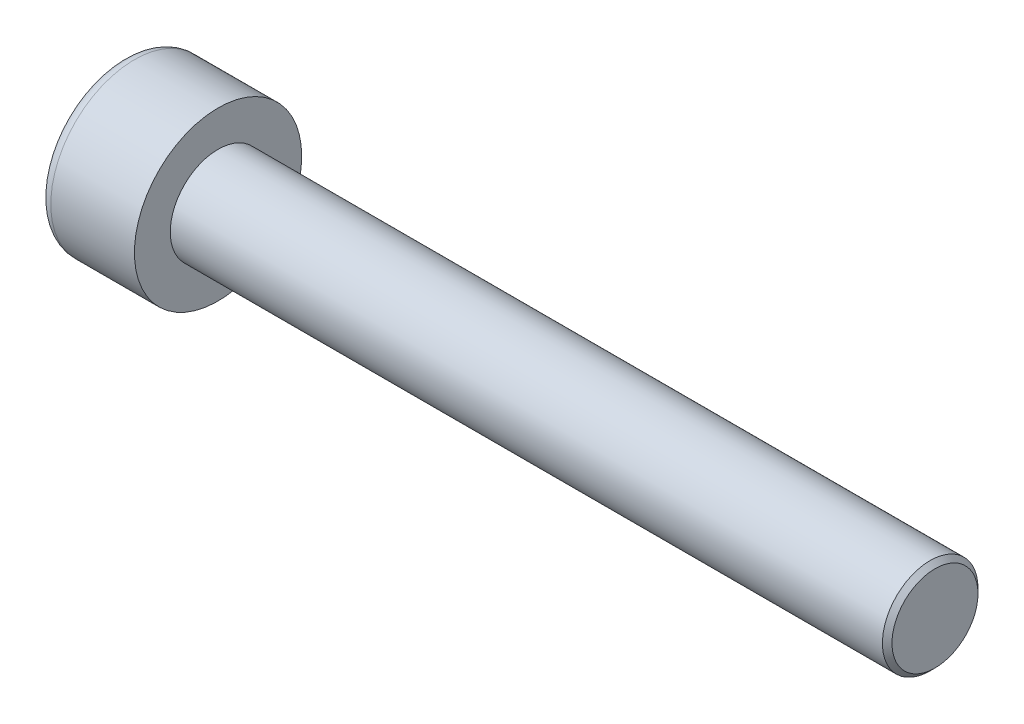
SolidWorks part; units mm, degrees
ref_plane "Front" through (0, 0, 0) normal (0, 0, 1) x (1, 0, 0)
ref_plane "Top" through (0, 0, 0) normal (0, 1, 0) x (1, 0, 0)
ref_plane "Right" through (0, 0, 0) normal (1, 0, 0) x (0, 0, -1)
sketch "Sketch1" plane through (0, 0, 0) normal (1, 0, 0) x (0, 0, -1)
  circle A0 centre (0, 0) radius 3.5
  dimension "dk" = 7
extrude "BaseHead" add sketch "Sketch1" along normal blind 4
sketch "Sketch2" plane through (4, 0, 0) normal (1, 0, 0) x (0, 0, -1)
  circle A0 centre (0, 0) radius 2
extrude "BaseBody" add sketch "Sketch2" along normal blind 30
cosmetic thread "ThreadCosmetic1" [suppressed] parameters "b"=20, "D2"=3.242
sketch "Sketch3" plane through (0, 0, 0) normal (1, 0, 0) x (0, 0, -1)
  line L1 (1.7321, 0) -> (0.866, 1.5)
  line L2 (0.866, 1.5) -> (-0.866, 1.5)
  line L3 (-0.866, 1.5) -> (-1.7321, 0)
  line L4 (-1.7321, 0) -> (-0.866, -1.5)
  line L5 (-0.866, -1.5) -> (0.866, -1.5)
  line L6 (0.866, -1.5) -> (1.7321, 0)
  circle A0 centre (0, 0) radius 1.5 construction
  dimension "s" = 3
  dimension "e" = 3.4641
extrude "HexagonSocket" cut sketch "Sketch3" along normal blind 2
sketch "Sketch4" plane through (-4.1961, 0.75, 0) normal (0, 0, 1) x (-1, 0, 0)
  line L0 (-6.1961, 2.25) -> (-7.0622, 0.75)
  line L2 (-7.0622, 0.75) -> (-6.1961, 0.75)
  line L3 (-6.1961, 0.75) -> (-6.1961, 2.25)
  line L4 (-5.0351, 0.75) -> (0.839, 0.75) construction
  line L5 (-38.1961, 0.75) -> (-8.1961, 0.75) construction
  line L6 (-8.1961, 0.75) -> (-4.1961, 0.75) construction
  dimension "m" = 60
revolve "Cut-Revolve1" cut sketch "Sketch4" angle 360 about L4
fillet "HeadFillet" [suppressed] radius 0.2
fillet "TopFillet" radius 0.5 1 edges at (0, 0, -3.5)
chamfer "Chamfer1" distance 0.2 angle 45 1 edges at (34, 0, -2)
sketch "Sketch5" plane through (0, 0, 0) normal (0, 0, 1) x (1, 0, 0)
  line L0 (33.8, 1.6718) -> (33.9895, 2)
  line L1 (33.9895, 2) -> (33.9895, 2.379)
  line L2 (33.9895, 2.379) -> (33.6105, 2.379)
  line L3 (33.6105, 2.379) -> (33.6105, 2)
  line L4 (33.6105, 2) -> (33.8, 1.6718)
  line L5 (0, 0) -> (7.8886, 0) construction
  line L6 (33.8, -2) -> (33.8, 2) construction
revolve "Cut-Revolve10" [suppressed] cut sketch "Sketch5" angle 360 about L5
pattern_linear "LPattern10" [suppressed] count 44 spacing 0.4548 along (1, 0, 0)
equation "\"r1@TopFillet\" = \"d@Sketch2\" / 8"
equation "\"D1@Chamfer1\" = \"r@HeadFillet\""
equation "\"D1@Sketch5\" = \"d@Sketch2\""
equation "\"D2@Sketch5\" =  ( \"d@Sketch2\" - \"D2@ThreadCosmetic1\" )  / 2"
equation "\"D3@LPattern10\" = \"D2@Sketch5\" * 1.2"
equation "\"D1@LPattern10\" = \"b@ThreadCosmetic1\" / \"D3@LPattern10\""
